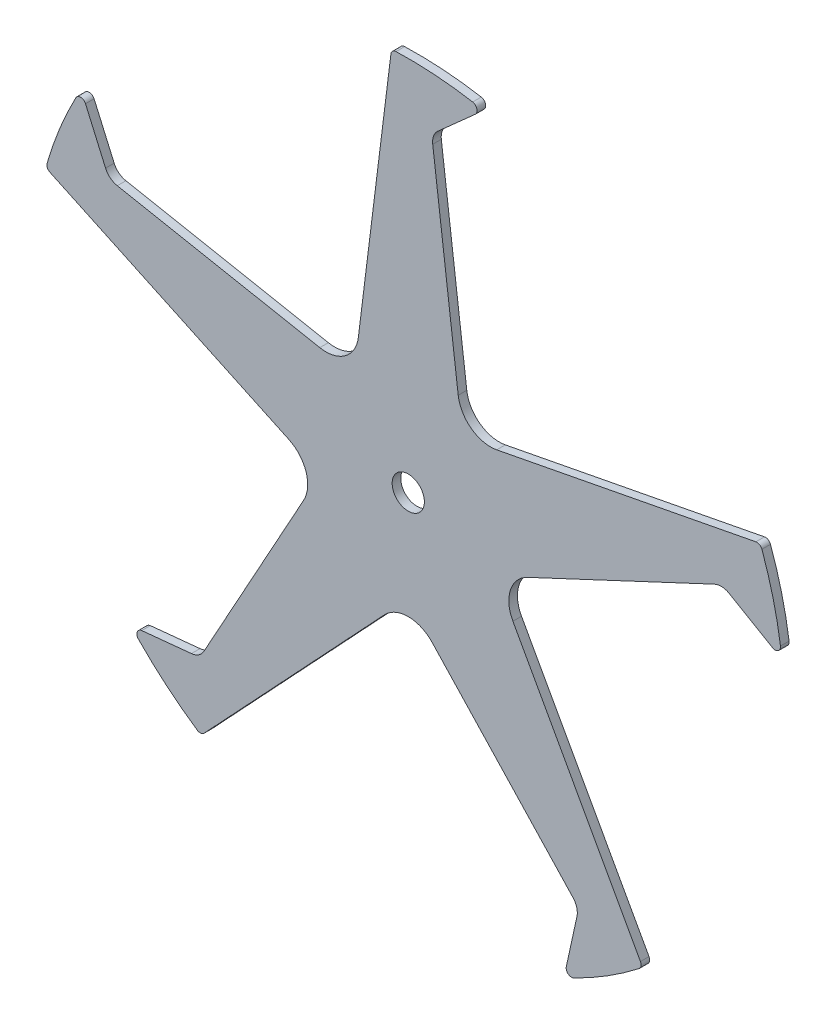
from build123d import *

# Parameters (mm, degrees)
SKETCH1_R               = 15
LINEAR_AUSTRAGEN1_DEPTH = 8


with BuildPart() as part:
    # Sketch1 → Linear austragen1 (new body)
    with BuildSketch(Plane.XY):
        with BuildLine():
            Line((-46.490516198, 101.722073941), (-16.145123023, 345.436482626))
            ThreePointArc((-16.145123023, 345.436482626), (-14.553663061, 348.512142372), (-11.345515054, 349.816064937))
            ThreePointArc((-11.345515054, 349.816064937), (24.425679263, 349.146654277), (59.941644882, 344.828941954))
            ThreePointArc((59.941644882, 344.828941954), (63.893687736, 341.27385411), (62.410890197, 336.16909126))
            Line((62.410890197, 336.16909126), (27.68409004, 305.238604713))
            ThreePointArc((27.68409004, 305.238604713), (23.620398385, 299.316491146), (22.775693358, 292.184065725))
            Line((22.775693358, 292.184065725), (46.490516198, 101.722073941))
            ThreePointArc((46.490516198, 101.722073941), (58.778525229, 80.901699437), (82.37708169, 75.648957927))
            Line((82.37708169, 75.648957927), (323.540500377, 122.100668066))
            ThreePointArc((323.540500377, 122.100668066), (326.957414795, 121.537530829), (329.188891102, 118.889334994))
            ThreePointArc((329.188891102, 118.889334994), (339.606150684, 84.662048273), (346.474799191, 49.550111254))
            ThreePointArc((346.474799191, 49.550111254), (344.314958136, 44.692912585), (339.001830525, 44.525678373))
            Line((339.001830525, 44.525678373), (298.854018333, 67.994781966))
            ThreePointArc((298.854018333, 67.994781966), (291.966003854, 70.02954866), (284.921635971, 68.628870213))
            Line((284.921635971, 68.628870213), (111.109800855, -12.781258825))
            ThreePointArc((111.109800855, -12.781258825), (95.10565163, -30.901699437), (97.402352577, -54.968446729))
            Line((97.402352577, -54.968446729), (216.104148993, -269.974119712))
            ThreePointArc((216.104148993, -269.974119712), (216.624458278, -273.397817411), (214.795438474, -276.338415011))
            ThreePointArc((214.795438474, -276.338415011), (185.462464648, -296.822630887), (154.191557264, -314.205289052))
            ThreePointArc((154.191557264, -314.205289052), (148.904659228, -313.652115076), (147.103763315, -308.650708653))
            Line((147.103763315, -308.650708653), (157.017850965, -263.215518401))
            ThreePointArc((157.017850965, -263.215518401), (156.824515556, -256.035849857), (153.315561803, -249.769091324))
            Line((153.315561803, -249.769091324), (22.179117214, -109.621326314))
            ThreePointArc((22.179117214, -109.621326314), (0, -100), (-22.179117214, -109.621326314))
            Line((-22.179117214, -109.621326314), (-189.980791189, -288.953850131))
            ThreePointArc((-189.980791189, -288.953850131), (-193.076136784, -290.506674439), (-196.438009496, -289.675867868))
            ThreePointArc((-196.438009496, -289.675867868), (-224.984043894, -268.108522791), (-251.179176024, -243.739659333))
            ThreePointArc((-251.179176024, -243.739659333), (-252.28681765, -238.540580345), (-248.086704923, -235.282306972))
            Line((-248.086704923, -235.282306972), (-201.811649597, -230.670918704))
            ThreePointArc((-201.811649597, -230.670918704), (-195.043122971, -228.26840621), (-190.167407773, -222.99465799))
            Line((-190.167407773, -222.99465799), (-97.402352577, -54.968446729))
            ThreePointArc((-97.402352577, -54.968446729), (-95.10565163, -30.901699437), (-111.109800855, -12.781258825))
            Line((-111.109800855, -12.781258825), (-333.518735158, 91.390819151))
            ThreePointArc((-333.518735158, 91.390819151), (-335.952073227, 93.854818649), (-336.200805025, 97.308882948))
            ThreePointArc((-336.200805025, 97.308882948), (-324.510250701, 131.122451129), (-309.428825313, 163.565895178))
            ThreePointArc((-309.428825313, 163.565895178), (-304.826487449, 166.225928727), (-300.429779115, 163.238245993))
            Line((-300.429779115, 163.238245993), (-281.744309741, 120.653050426))
            ThreePointArc((-281.744309741, 120.653050426), (-277.367794824, 114.958216262), (-270.845483359, 111.950813376))
            Line((-270.845483359, 111.950813376), (-82.37708169, 75.648957927))
            ThreePointArc((-82.37708169, 75.648957927), (-58.778525229, 80.901699437), (-46.490516198, 101.722073941))
        make_face()
        Circle(SKETCH1_R, mode=Mode.SUBTRACT)
    extrude(amount=LINEAR_AUSTRAGEN1_DEPTH)


solid = part.part
